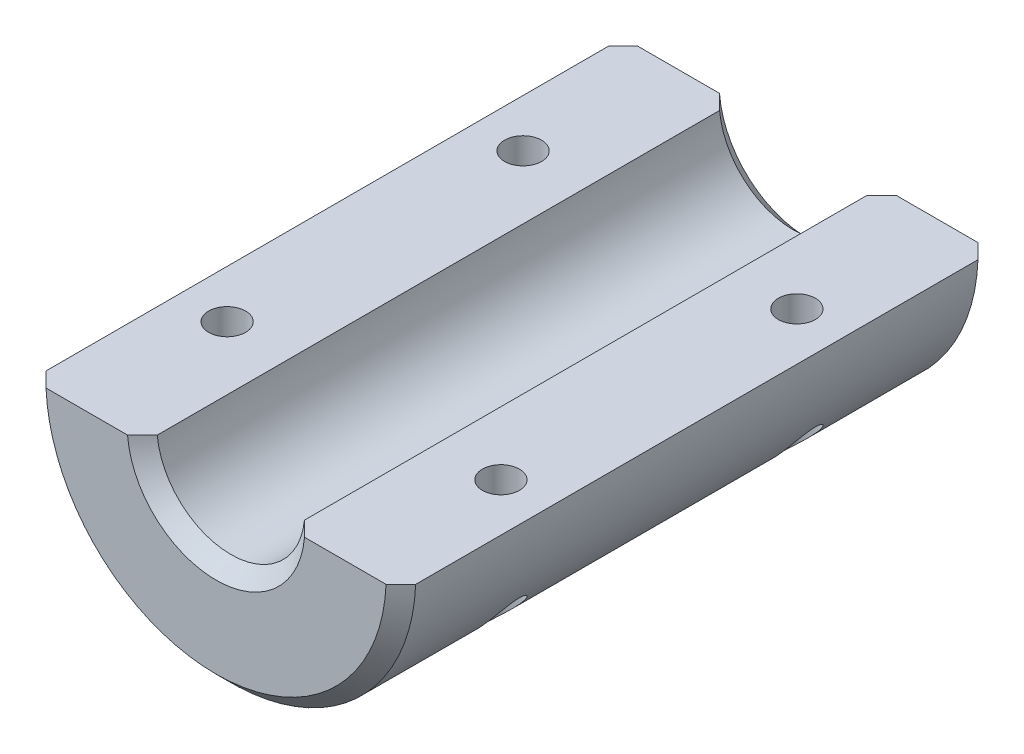
from build123d import *

# Parameters (mm, degrees)
EXTRUDE_1_DEPTH    = 80
HOLE_WIZARD_M6_1_D = 5
CHAMFER_1_SIZE     = 2


with BuildPart() as part:
    # 草图1 → 凸台-拉伸1 (new body)
    with BuildSketch(Plane.XY):
        with BuildLine():
            Line((-24.979991994, -1), (-9.949874371, -1))
            ThreePointArc((-9.949874371, -1), (0, -10), (9.949874371, -1))
            Line((9.949874371, -1), (24.979991994, -1))
            ThreePointArc((24.979991994, -1), (0, -25), (-24.979991994, -1))
        make_face()
    extrude(amount=EXTRUDE_1_DEPTH)

    # M6 螺纹孔1 (through all)
    with Locations(Plane(origin=(0, -1, 0), x_dir=(1, 0, 0), z_dir=(0, 1, 0))):
        with Locations((-18.5, -20), (18.5, -20), (18.5, -60), (-18.5, -60)):
            Hole(HOLE_WIZARD_M6_1_D / 2)

    # 倒角1
    chamfer_1_edges = [part.edges().sort_by_distance(p)[0] for p in [
        (0, -25, 80),
        (0, -10, 80),
        (0, -25, 0),
        (0, -10, 0),
    ]]
    chamfer(chamfer_1_edges, length=CHAMFER_1_SIZE)


solid = part.part
